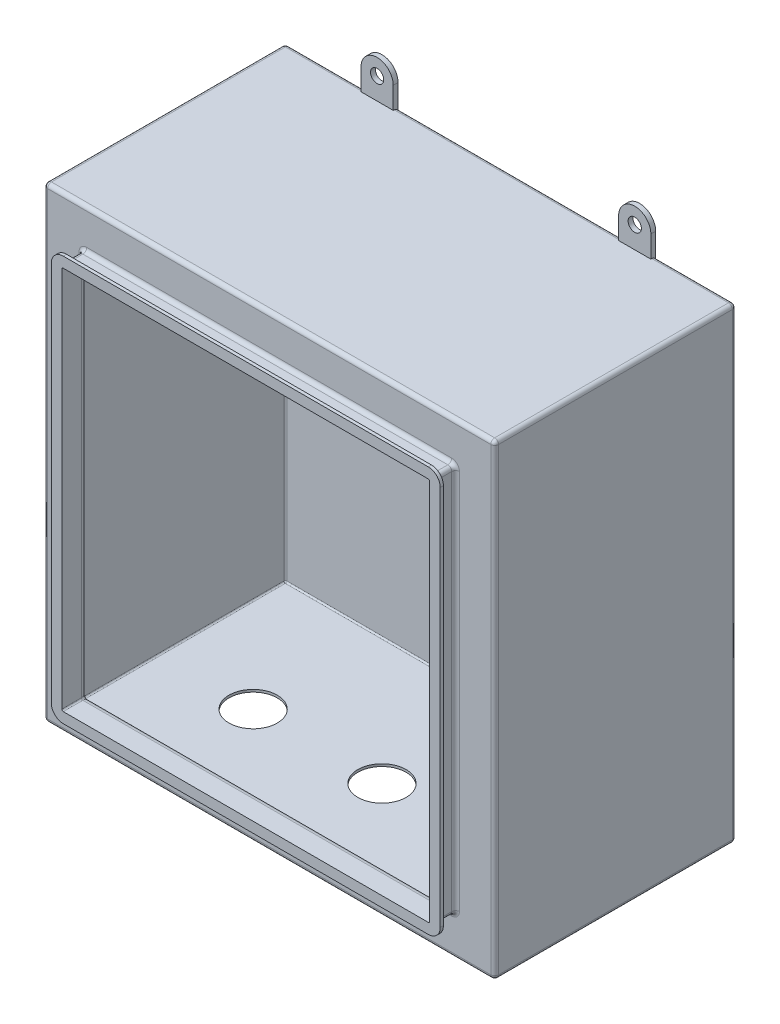
SolidWorks part; units mm, degrees
material "普通碳钢"
ref_plane "前视基准面" through (0, 0, 0) normal (0, 0, 1) x (1, 0, 0)
ref_plane "上视基准面" through (0, 0, 0) normal (0, 1, 0) x (1, 0, 0)
ref_plane "右视基准面" through (0, 0, 0) normal (1, 0, 0) x (0, 0, -1)
sketch "草图1" plane through (0, 0, 0) normal (0, 1, 0) x (1, 0, 0)
  line L1 (-140, -75) -> (140, -75)
  line L2 (-140, -75) -> (-140, 75)
  line L3 (-140, 75) -> (140, 75)
  line L4 (140, -75) -> (140, 75)
  line L5 (-140, -75) -> (140, 75) construction
  line L6 (-140, 75) -> (140, -75) construction
  point P0 (0, 0)
  dimension "D1" = 280
  dimension "D2" = 150
extrude "凸台-拉伸1" add sketch "草图1" along normal blind 290
fillet "圆角1" radius 2.4 12 edges at (0, 290, 75) (-140, 290, 0) (-140, 0, 0) (0, 0, 75) (0, 290, -75) (-140, 145, -75) (0, 0, -75) (140, 145, 75) (140, 290, 0) (140, 145, -75) (140, 0, 0) (-140, 145, 75)
sketch "草图2" plane through (0, 0, 75) normal (0, 0, 1) x (1, 0, 0)
  line L0 (137.6, 0) -> (-137.6, 0) construction
  line L1 (-115.74, 265.74) -> (115.74, 265.74)
  line L2 (-115.74, 265.74) -> (-115.74, 24.26)
  line L3 (-115.74, 24.26) -> (115.74, 24.26)
  line L4 (115.74, 265.74) -> (115.74, 24.26)
  line L5 (140, 287.6) -> (140, 2.4) construction
  line L6 (-140, 2.4) -> (-140, 287.6) construction
  dimension "D1" = 24.26
  dimension "D2" = 24.26
  dimension "D3" = 24.26
  dimension "D4" = 241.48
extrude "凸台-拉伸2" add sketch "草图2" along normal blind 14.57
fillet "圆角2" radius 2.4 8 edges at (0, 24.26, 75) (115.74, 145, 75) (-115.74, 24.26, 82.285) (115.74, 24.26, 82.285) (115.74, 265.74, 82.285) (-115.74, 265.74, 82.285) (0, 265.74, 75) (-115.74, 145, 75)
shell "抽壳1" thickness 1.5
sketch "草图3" plane through (0, 1.5, 0) normal (0, 1, 0) x (1, 0, 0)
  line L1 (137.6, 75) -> (-137.6, 75) construction
  line L2 (-140, 72.6) -> (-140, -72.6) construction
  circle A0 centre (-80, -5) radius 15
  circle A17 centre (0, -5) radius 15
  circle A18 centre (80, -5) radius 15
  dimension "D1" = 30
  dimension "D2" = 3
  dimension "D7" = 80
  dimension "D8" = 60
extrude "切除-拉伸1" cut sketch "草图3" against normal through all
sketch "草图4" plane through (0, 0, -75) normal (0, 0, -1) x (-1, 0, 0)
  line L1 (-205.123, 145) -> (354.4087, 145) construction
  line L7 (140, 287.6) -> (140, 2.4) construction
  line L8 (-90, 288.5) -> (-70, 288.5)
  line L13 (-90, 1.5) -> (-90, -13.5)
  line L20 (70, 1.5) -> (70, -13.5)
  line L25 (90, -13.5) -> (90, 1.5)
  line L26 (70, 1.5) -> (90, 1.5)
  line L27 (-70, -13.5) -> (-70, 1.5)
  line L28 (-90, 1.5) -> (-70, 1.5)
  line L29 (-140, 2.4) -> (-140, 287.6) construction
  line L30 (137.6, 0) -> (-137.6, 0) construction
  line L31 (-70, 303.5) -> (-70, 288.5)
  line L36 (70, 288.5) -> (90, 288.5)
  line L37 (90, 303.5) -> (90, 288.5)
  line L38 (70, 288.5) -> (70, 303.5)
  line L39 (-90, 288.5) -> (-90, 303.5)
  arc A10 (70, -13.5) -> (90, -13.5) centre (80, -13.5) ccw
  circle A11 centre (80, -13.5) radius 4.1
  arc A12 (-90, -13.5) -> (-70, -13.5) centre (-80, -13.5) ccw
  circle A13 centre (-80, -13.5) radius 4.1
  circle A16 centre (-80, 303.5) radius 4.1
  arc A17 (-90, 303.5) -> (-70, 303.5) centre (-80, 303.5) cw
  circle A18 centre (80, 303.5) radius 4.1
  arc A19 (70, 303.5) -> (90, 303.5) centre (80, 303.5) cw
  dimension "D2" = 8.2
  dimension "D4" = 0
  dimension "D10" = 50
  dimension "D13" = 15
  dimension "D8" = 8.2
  dimension "D17" = 10
  dimension "D18" = 10
  dimension "D3" = 50
  dimension "D5" = 1.5
  dimension "D9" = 15
  dimension "D11" = 15
  dimension "D12" = 15
  dimension "D19" = 145
extrude "凸台-拉伸3" add sketch "草图4" against normal blind 3
sketch "草图5" plane through (0, 0, 89.57) normal (0, 0, 1) x (1, 0, 0)
  line L0 (-120.74, 263.34) -> (-120.74, 26.66)
  line L1 (-113.34, 19.26) -> (113.34, 19.26)
  line L2 (120.74, 26.66) -> (120.74, 263.34)
  line L3 (113.34, 270.74) -> (-113.34, 270.74)
  line L4 (-115.74, 263.34) -> (-115.74, 26.66)
  line L5 (-113.34, 24.26) -> (113.34, 24.26)
  line L6 (115.74, 26.66) -> (115.74, 263.34)
  line L7 (113.34, 265.74) -> (-113.34, 265.74)
  line L8 (-115.74, 263.34) -> (-115.74, 26.66)
  line L9 (-113.34, 24.26) -> (113.34, 24.26)
  line L10 (115.74, 26.66) -> (115.74, 263.34)
  line L11 (113.34, 265.74) -> (-113.34, 265.74)
  arc A0 (-120.74, 26.66) -> (-113.34, 19.26) centre (-113.34, 26.66) ccw
  arc A1 (113.34, 19.26) -> (120.74, 26.66) centre (113.34, 26.66) ccw
  arc A2 (120.74, 263.34) -> (113.34, 270.74) centre (113.34, 263.34) ccw
  arc A3 (-113.34, 270.74) -> (-120.74, 263.34) centre (-113.34, 263.34) ccw
  arc A4 (-115.74, 26.66) -> (-113.34, 24.26) centre (-113.34, 26.66) ccw
  arc A5 (113.34, 24.26) -> (115.74, 26.66) centre (113.34, 26.66) ccw
  arc A6 (115.74, 263.34) -> (113.34, 265.74) centre (113.34, 263.34) ccw
  arc A7 (-113.34, 265.74) -> (-115.74, 263.34) centre (-113.34, 263.34) ccw
  arc A8 (-115.74, 26.66) -> (-113.34, 24.26) centre (-113.34, 26.66) ccw
  arc A9 (113.34, 24.26) -> (115.74, 26.66) centre (113.34, 26.66) ccw
  arc A10 (115.74, 263.34) -> (113.34, 265.74) centre (113.34, 263.34) ccw
  arc A11 (-113.34, 265.74) -> (-115.74, 263.34) centre (-113.34, 263.34) ccw
  dimension "D1" = 0
  dimension "D2" = 5
extrude "凸台-拉伸4" add sketch "草图5" against normal blind 2
